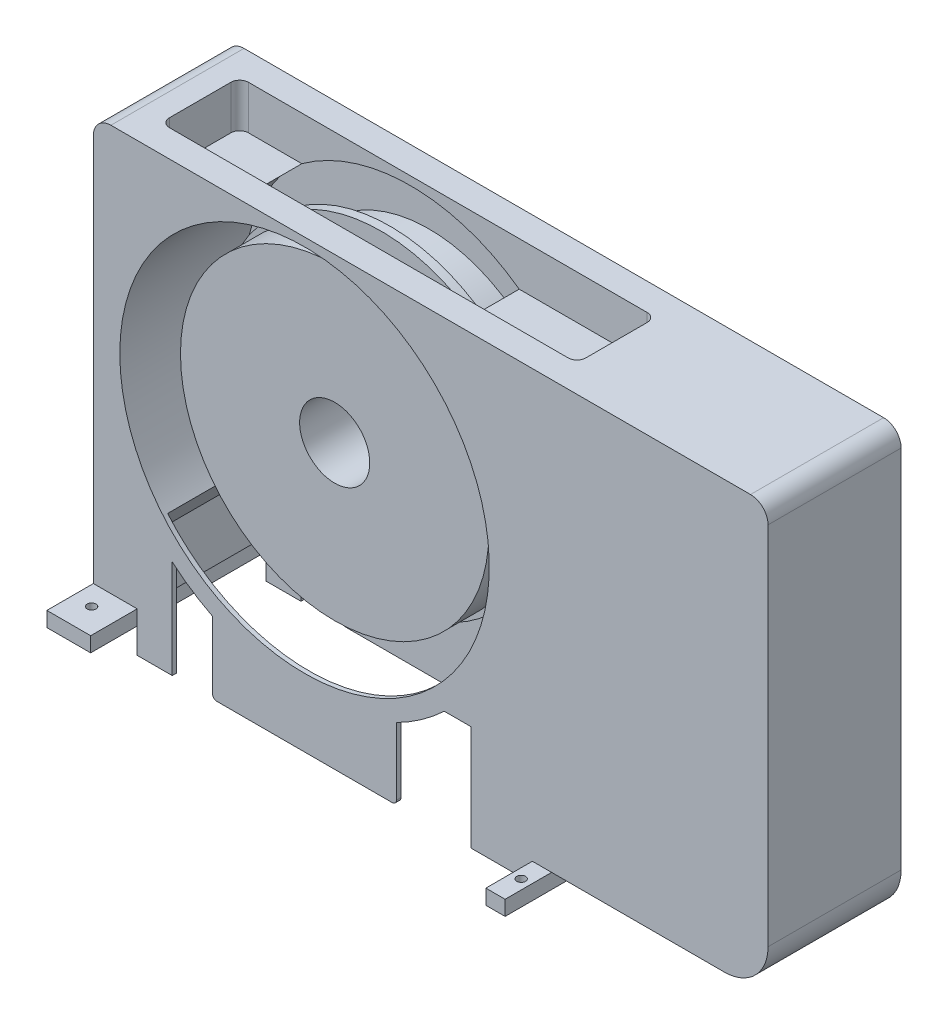
SolidWorks part; units mm, degrees
ref_plane "Front Plane" through (0, 0, 0) normal (0, 0, 1) x (1, 0, 0)
ref_plane "Top Plane" through (0, 0, 0) normal (0, 1, 0) x (1, 0, 0)
ref_plane "Right Plane" through (0, 0, 0) normal (1, 0, 0) x (0, 0, -1)
other "Configuration Table"
sketch "Sketch1" plane through (0, 318.5, 0) normal (0, -1, 0) x (-1, 0, 0)
  line L0 (0, 0) -> (0, 229.4548) construction
  line L1 (30, 87.5) -> (-30, 87.5) construction
  line L2 (-176, 125.5) -> (-167.6756, 125.5)
  line L3 (-176, 125.5) -> (-176, 87.5)
  line L4 (-176, 87.5) -> (-40, 87.5)
  line L5 (-40, 150.5) -> (-40, 87.5)
  line L6 (91.8, 125.5) -> (46.8, 125.5) construction
  line L7 (-157.6756, 120.5) -> (-157.6756, 140.5)
  line L8 (-157.6756, 140.5) -> (-182.6756, 140.5)
  line L9 (-182.6756, 140.5) -> (-182.6756, 150.5)
  line L10 (-182.6756, 150.5) -> (-40, 150.5)
  line L11 (-167.6756, 125.5) -> (-167.6756, 120.5)
  line L12 (-167.6756, 120.5) -> (-157.6756, 120.5)
  dimension "D1" = 176
  dimension "D2" = 40
  dimension "D3" = 25
  dimension "D4" = 10
  dimension "D5" = 157.6756
  dimension "D6" = 10
  dimension "D7" = 5
  dimension "D8" = 20
revolve "Revolve1" add sketch "Sketch1" angle 360 about L0
sketch "Sketch2" plane through (0, 0, 0) normal (0, 0, 1) x (1, 0, 0)
  line L0 (-191, 59) -> (-241, 59)
  line L1 (-241, 59) -> (-241, 76)
  line L3 (260, 52) -> (282, 52)
  line L5 (260, 35) -> (282, 35)
  line L6 (282, 35) -> (282, 52)
  line L9 (-241, 76) -> (-191, 76)
  line L10 (260, 35) -> (260, 52)
  line L11 (-191, 59) -> (-191, 76)
  dimension "D1" = 17
  dimension "D2" = 17
extrude "Boss-Extrude1" add sketch "Sketch2" against normal blind 205 separate body
sketch "Sketch3" plane through (0, 0, -53.1) normal (0, 0, -1) x (-1, 0, 0)
  line L0 (-529, 539) -> (241, 539)
  line L1 (241, 59) -> (191, 59) construction
  line L2 (241, 539) -> (241, 76)
  line L3 (-282, 529) -> (-282, 76)
  line L4 (241, 76) -> (241, 59) construction
  line L5 (-282, 35) -> (-282, 52) construction
  line L6 (-529, 52) -> (-260, 52)
  line L7 (189.3118, 76) -> (241, 76)
  line L8 (191, 76) -> (241, 76) construction
  line L9 (-282, 52) -> (-260, 52) construction
  line L10 (189.3118, 76) -> (189.3118, 143.5627)
  line L11 (189.3118, 143.5627) -> (161.2521, 182.6609)
  line L12 (-260, 52) -> (-260, 205.9418)
  line L13 (-260, 205.9418) -> (-195.1184, 238.6044)
  line L14 (185.6394, 174.4062) -> (207.8757, 143.4222)
  line L15 (226, 149.2528) -> (226, 254.0873)
  line L16 (-529, 539) -> (-529, 52)
  line L17 (-519, 529) -> (-519, 76)
  line L18 (-282, 529) -> (-519, 529)
  line L19 (-282, 76) -> (-519, 76)
  arc A0 (161.2521, 182.6609) -> (-195.1184, 238.6044) centre (0, 318.5) ccw
  arc A1 (30.2283, 520.0886) -> (22.9766, 521.0433) centre (0, 318.5) ccw construction
  arc A2 (226, 149.2528) -> (207.8757, 143.4222) centre (216, 149.2528) cw
  arc A3 (185.6394, 174.4062) -> (226, 254.0873) centre (0, 318.5) ccw
  dimension "D2" = 7
  dimension "D5" = 10
  dimension "D6" = 235
  dimension "D1" = 480
  dimension "D3" = 15
  dimension "D4" = 15
  dimension "D7" = 10
  dimension "D8" = 10
  dimension "D9" = 770
extrude "Boss-Extrude2" add sketch "Sketch3" along normal blind 151.9
sketch "Sketch4" plane through (0, 0, -205) normal (0, 0, -1) x (-1, 0, 0)
  line L0 (-196.9102, 237.7024) -> (-147.4365, 262.6083)
  line L1 (-260, 205.9418) -> (-195.1184, 238.6044) construction
  line L2 (162.4547, 180.9852) -> (128.9173, 227.716)
  line L3 (161.2521, 182.6609) -> (189.3118, 143.5627) construction
  arc A0 (128.9173, 227.716) -> (-147.4365, 262.6083) centre (0, 318.5) ccw
  arc A1 (161.2521, 182.6609) -> (-195.1184, 238.6044) centre (0, 318.5) ccw construction
  arc A2 (161.2521, 182.6609) -> (-195.1184, 238.6044) centre (0, 318.5) ccw construction
  arc A3 (-196.9102, 237.7024) -> (162.4547, 180.9852) centre (0, 318.5) cw
  dimension "D1" = 157.675
  dimension "D2" = 2
extrude "Boss-Extrude3" add sketch "Sketch4" against normal blind 10
sketch "Sketch5" plane through (0, 0, -205) normal (0, 0, -1) x (-1, 0, 0)
  line L1 (-519, 529) -> (-282, 529)
  line L2 (-519, 529) -> (-519, 76)
  line L3 (-519, 76) -> (-282, 76)
  line L4 (-282, 529) -> (-282, 76)
extrude "Boss-Extrude4" add sketch "Sketch5" against normal blind 5
sketch "Sketch6" plane through (0, 0, -53.1) normal (0, 0, 1) x (1, 0, 0)
  line L4 (519, 76) -> (519, 529)
  line L5 (519, 529) -> (282, 529)
  line L6 (282, 529) -> (282, 76)
  line L7 (282, 76) -> (519, 76)
  line L8 (519, 76) -> (519, 529)
  line L9 (519, 529) -> (282, 529)
  line L10 (282, 529) -> (282, 76)
  line L11 (282, 76) -> (519, 76)
  dimension "D1" = 0
extrude "Boss-Extrude5" add sketch "Sketch6" against normal blind 5
sketch "Sketch8" plane through (0, 0, -205) normal (0, 0, -1) x (-1, 0, 0)
  line L0 (-190, 30) -> (-190, 150) construction
  line L1 (-190, 150) -> (-120, 150) construction
  line L2 (-105, 135) -> (-105, 35) construction
  line L3 (-120, 150) -> (-105, 135) construction
  line L6 (-190, 30) -> (-190, 150)
  line L7 (-190, 150) -> (-120, 150)
  line L8 (-105, 135) -> (-105, 35)
  line L9 (-120, 150) -> (-105, 135)
  line L12 (120, 150) -> (151, 150) construction
  line L13 (151, 150) -> (151, 30) construction
  line L16 (120, 150) -> (151, 150)
  line L17 (151, 150) -> (151, 30)
  line L21 (105, 35) -> (105, 135) construction
  line L22 (105, 135) -> (120, 150) construction
  line L24 (105, 35) -> (105, 135)
  line L25 (105, 135) -> (120, 150)
  line L30 (191, 30) -> (191, 59) construction
  line L32 (191, 30) -> (191, 59)
  line L34 (191, 59) -> (191, 76) construction
  line L35 (191, 59) -> (191, 76)
  line L36 (189.3118, 76) -> (191, 76)
  line L37 (-260, 205.9418) -> (-148.6486, 261.9982)
  line L38 (189.3118, 76) -> (189.3118, 143.5627)
  line L39 (129.7501, 226.5556) -> (189.3118, 143.5627)
  line L40 (-100, 30) -> (100, 30)
  line L41 (151, 30) -> (191, 30)
  line L42 (-260, 205.9418) -> (-260, 30)
  line L43 (-190, 30) -> (-260, 30)
  arc A0 (-105, 35) -> (-100, 30) centre (-100, 35) ccw construction
  arc A2 (-105, 35) -> (-100, 30) centre (-100, 35) ccw
  arc A4 (-148.6486, 261.9982) -> (129.7501, 226.5556) centre (0, 318.5) ccw
  arc A5 (100, 30) -> (105, 35) centre (100, 35) ccw
extrude "Boss-Extrude7" add sketch "Sketch8" against normal blind 5
sketch "Sketch9" plane through (0, 0, -53.1) normal (0, 0, 1) x (1, 0, 0)
  line L0 (-185.6394, 174.4062) -> (-207.8757, 143.4222) construction
  line L1 (-226, 149.2528) -> (-226, 254.0873) construction
  line L2 (-189.3118, 143.5627) -> (-189.3118, 76) construction
  line L3 (-161.2521, 182.6609) -> (-189.3118, 143.5627) construction
  line L4 (260, 52) -> (260, 205.9418) construction
  line L5 (260, 205.9418) -> (195.1184, 238.6044) construction
  line L6 (-185.6394, 174.4062) -> (-207.8757, 143.4222)
  line L7 (-226, 149.2528) -> (-226, 254.0873)
  line L8 (-189.3118, 143.5627) -> (-189.3118, 76)
  line L9 (-161.2521, 182.6609) -> (-189.3118, 143.5627)
  line L10 (260, 52) -> (260, 205.9418)
  line L11 (260, 205.9418) -> (195.1184, 238.6044)
  line L16 (190, 150) -> (159.4734, 150) construction
  line L21 (190, 150) -> (159.4734, 150)
  line L22 (-191, 30) -> (-191, 59) construction
  line L24 (-191, 30) -> (-191, 76)
  line L26 (-189.3118, 76) -> (-191, 76) construction
  line L27 (-189.3118, 76) -> (-191, 76)
  line L28 (260, 52) -> (260, 35) construction
  line L29 (260, 35) -> (260, 30) construction
  line L30 (260, 30) -> (-191, 30) construction
  line L32 (260, 52) -> (260, 35)
  line L33 (260, 35) -> (260, 30)
  line L34 (260, 30) -> (190, 30)
  line L36 (-191, 30) -> (-151, 30)
  line L37 (-151, 30) -> (-151, 142.3665)
  line L38 (-105, 111.6208) -> (-105, 35)
  line L39 (-100, 30) -> (100, 30)
  line L40 (105, 111.6208) -> (105, 35)
  line L41 (190, 150) -> (190, 30)
  arc A0 (-226, 254.0873) -> (-185.6394, 174.4062) centre (0, 318.5) ccw construction
  arc A1 (-226, 149.2528) -> (-207.8757, 143.4222) centre (-216, 149.2528) ccw construction
  arc A2 (-226, 254.0873) -> (-185.6394, 174.4062) centre (0, 318.5) ccw
  arc A3 (-226, 149.2528) -> (-207.8757, 143.4222) centre (-216, 149.2528) ccw
  arc A4 (-151, 142.3665) -> (-105, 111.6208) centre (0, 318.5) ccw construction
  arc A5 (105, 111.6208) -> (159.4734, 150) centre (0, 318.5) ccw construction
  arc A6 (-151, 142.3665) -> (-105, 111.6208) centre (0, 318.5) ccw
  arc A7 (105, 111.6208) -> (159.4734, 150) centre (0, 318.5) ccw
  arc A12 (-161.2521, 182.6609) -> (195.1184, 238.6044) centre (0, 318.5) ccw
  arc A13 (-100, 30) -> (-105, 35) centre (-100, 35) cw
  arc A14 (100, 30) -> (105, 35) centre (100, 35) ccw
  dimension "D2" = 5
extrude "Boss-Extrude8" add sketch "Sketch9" against normal blind 5
sketch "Sketch10" plane through (0, 0, -205) normal (0, 0, -1) x (-1, 0, 0)
  line L0 (226, 149.2528) -> (226, 254.0873) construction
  line L1 (226, 149.2528) -> (226, 254.0873)
  line L2 (185.6394, 174.4062) -> (207.8757, 143.4222) construction
  line L3 (185.6394, 174.4062) -> (207.8757, 143.4222)
  arc A0 (185.6394, 174.4062) -> (226, 254.0873) centre (0, 318.5) ccw construction
  arc A1 (185.6394, 174.4062) -> (226, 254.0873) centre (0, 318.5) ccw
  arc A2 (207.8757, 143.4222) -> (226, 149.2528) centre (216, 149.2528) ccw construction
  arc A3 (207.8757, 143.4222) -> (226, 149.2528) centre (216, 149.2528) ccw
extrude "Boss-Extrude9" add sketch "Sketch10" against normal blind 5
fillet "Fillet1" radius 20 2 edges at (-241, 539, -129.05) (529, 539, -129.05)
fillet "Fillet2" radius 50 1 edges at (529, 52, -129.05)
sketch "Sketch12" plane through (0, 539, 0) normal (0, 1, 0) x (1, 0, 0)
  line L4 (-185, 174.05) -> (270, 174.05)
  line L5 (280, 164.05) -> (280, 94.05)
  line L6 (270, 84.05) -> (-185, 84.05)
  line L7 (-195, 94.05) -> (-195, 164.05)
  line L10 (295, 79.05) -> (295, 179.05) construction
  line L11 (285, 189.05) -> (-200, 189.05) construction
  line L12 (-200, 69.05) -> (285, 69.05) construction
  line L13 (-210, 179.05) -> (-210, 79.05) construction
  arc A0 (270, 174.05) -> (280, 164.05) centre (270, 164.05) cw
  arc A1 (280, 94.05) -> (270, 84.05) centre (270, 94.05) cw
  arc A2 (-185, 84.05) -> (-195, 94.05) centre (-185, 94.05) cw
  arc A3 (-195, 164.05) -> (-185, 174.05) centre (-185, 164.05) cw
  dimension "D1" = 10
  dimension "D2" = 10
  dimension "D3" = 10
  dimension "D4" = 10
  dimension "D5" = 15
  dimension "D6" = 15
  dimension "D7" = 15
  dimension "D8" = 15
extrude "Cut-Extrude1" cut sketch "Sketch12" against normal blind 50
sketch "Sketch13" plane through (0, 0, -205) normal (0, 0, -1) x (-1, 0, 0)
  line L4 (191, 76) -> (191, 59)
  line L5 (241, 76) -> (191, 76)
  line L6 (241, 59) -> (241, 76)
  line L7 (191, 59) -> (241, 59)
  line L8 (191, 76) -> (191, 59)
  line L9 (241, 76) -> (191, 76)
  line L10 (241, 59) -> (241, 76)
  line L11 (191, 59) -> (241, 59)
  line L12 (-260, 35) -> (-260, 52)
  line L13 (-282, 35) -> (-260, 35)
  line L14 (-282, 52) -> (-282, 35)
  line L15 (-260, 52) -> (-282, 52)
  line L16 (-260, 35) -> (-260, 52)
  line L17 (-282, 35) -> (-260, 35)
  line L18 (-282, 52) -> (-282, 35)
  line L19 (-260, 52) -> (-282, 52)
  dimension "D1" = 0
  dimension "D2" = 0
extrude "Boss-Extrude10" add sketch "Sketch13" along normal blind 30
sketch "Sketch14" plane through (0, 76, 0) normal (0, 1, 0) x (1, 0, 0)
  line L0 (271, 235) -> (271, 262.8214) construction
  line L1 (260, 235) -> (282, 235) construction
  circle A0 centre (-219.3032, 219.9981) radius 5
  circle A1 centre (-219.3032, 29.3637) radius 5
  circle A2 centre (271, 219.9981) radius 5
  circle A3 centre (271, 29.3637) radius 5
  dimension "D1" = 10
extrude "Cut-Extrude2" cut sketch "Sketch14" against normal through all
sketch "Sketch16" plane through (0, 0, -150.5) normal (0, 0, -1) x (-1, 0, 0)
  circle A0 centre (0, 318.5) radius 157.675
  arc A1 (128.9173, 227.716) -> (-147.4365, 262.6083) centre (0, 318.5) ccw construction
  circle A2 centre (0, 318.5) radius 52
  dimension "D1" = 104
extrude "Boss-Extrude12" add sketch "Sketch16" along normal blind 54.4
